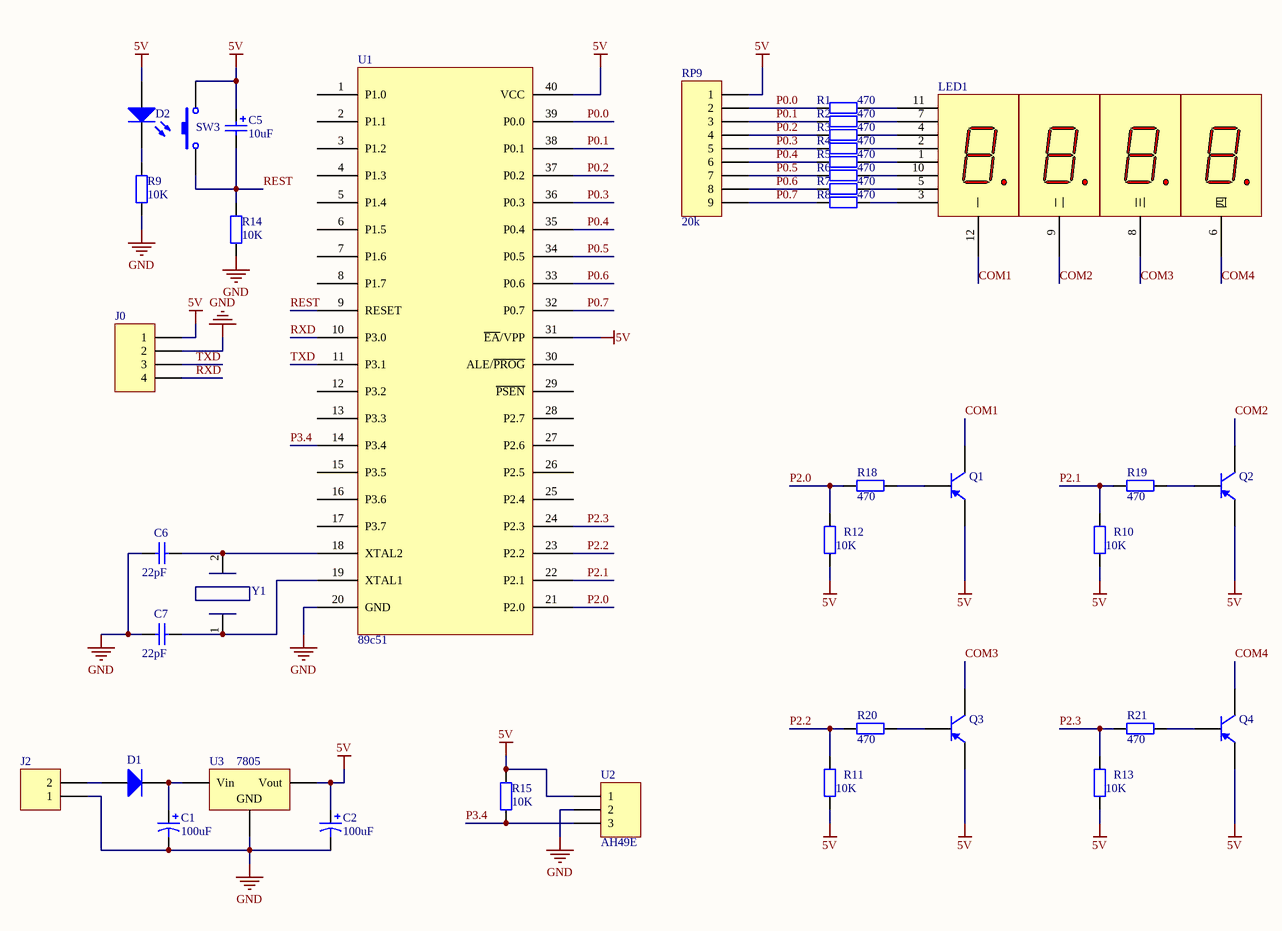
[diagram p0: MISC89328.SchDoc]
# Altium project MISC89328.PrjPcb
1 sheet, 39 parts. Net scope: global (net labels, ports and power ports of the same name join across sheets).
Board files: MISC89328.PcbDoc, MISC89328-28.PcbDoc

## Sheet MISC89328.SchDoc
size A3

### Parts
C1  100uF  [RB7.6-15]
C2  value 100uF  [RB7.6-15]  (hidden comment: Cap Pol1)
C5  value 10uF  [POLAR0.8]  (hidden comment: Cap Pol2)
C6  value 22pF  [RAD-0.3]  (hidden comment: Cap)
C7  value 22pF  [RAD-0.3]  (hidden comment: Cap)
D1  Diode 1N914  [DO-35]  (value not drawn)
D2  LED0  [LED-0]  (value not drawn)
J0  Header 4  [HDR1X4]  (value not drawn)
J2  Header 2  [HDR1X2]  (value not drawn)
LED1  Dpy Red-CA  [四位数码管]  (value not drawn)
Q1  2N3906  [TO-92A]  (value not drawn)
Q2  2N3906  [TO-92A]  (value not drawn)
Q3  2N3906  [TO-92A]  (value not drawn)
Q4  2N3906  [TO-92A]  (value not drawn)
R1  value 470  [AXIAL-0.4]  (hidden comment: Res2)
R2  value 470  [AXIAL-0.4]  (hidden comment: Res2)
R3  value 470  [AXIAL-0.4]  (hidden comment: Res2)
R4  value 470  [AXIAL-0.4]  (hidden comment: Res2)
R5  value 470  [AXIAL-0.4]  (hidden comment: Res2)
R6  value 470  [AXIAL-0.4]  (hidden comment: Res2)
R7  value 470  [AXIAL-0.4]  (hidden comment: Res2)
R8  value 470  [AXIAL-0.4]  (hidden comment: Res2)
R9  value 10K  [AXIAL-0.4]  (hidden comment: Res2)
R10  value 10K  [AXIAL-0.4]  (hidden comment: Res2)
R11  value 10K  [AXIAL-0.4]  (hidden comment: Res2)
R12  value 10K  [AXIAL-0.4]  (hidden comment: Res2)
R13  value 10K  [AXIAL-0.4]  (hidden comment: Res2)
R14  value 10K  [AXIAL-0.4]  (hidden comment: Res2)
R15  value 10K  [AXIAL-0.4]  (hidden comment: Res2)
R18  value 470  [AXIAL-0.4]  (hidden comment: Res2)
R19  value 470  [AXIAL-0.4]  (hidden comment: Res2)
R20  value 470  [AXIAL-0.4]  (hidden comment: Res2)
R21  value 470  [AXIAL-0.4]  (hidden comment: Res2)
RP9  20k  [HDR1X9]
SW3  SW-PB  [SPST-2]  (value not drawn)
U1  89c51  [89c51]
U2  AH49E  [HDR1X3]
U3  7805  [PCBComponent_1]
Y1  Component_1  [LC-HC-49S]  (value not drawn)

### Nets
5V: C2.1 C5.1 D2.1(A) J0.1 Q1.1(E) Q2.1(E) Q3.1(E) Q4.1(E) R10.1 R11.1 R12.1 R13.1 R15.2 RP9.1 SW3.2 U1.31(~{EA}/VPP) U1.40(VCC) U2.1 U3.3(Vout)
GND: C1.2 C2.2 C6.2 C7.2 J0.2 J2.1 R9.2 R14.2 U1.20(GND) U2.2 U3.2(GND)
COM1: LED1.12(一) Q1.3(C)
COM2: LED1.9(二) Q2.3(C)
COM3: LED1.8(三) Q3.3(C)
COM4: LED1.6(四) Q4.3(C)
P0.0: R1.1 RP9.2 U1.39(P0.0)
P0.1: R2.1 RP9.3 U1.38(P0.1)
P0.2: R3.1 RP9.4 U1.37(P0.2)
P0.3: R4.1 RP9.5 U1.36(P0.3)
P0.4: R5.1 RP9.6 U1.35(P0.4)
P0.5: R6.1 RP9.7 U1.34(P0.5)
P0.6: R7.1 RP9.8 U1.33(P0.6)
P0.7: R8.1 RP9.9 U1.32(P0.7)
P2.0: R12.2 R18.2 U1.21(P2.0)
P2.1: R10.2 R19.2 U1.22(P2.1)
P2.2: R11.2 R20.2 U1.23(P2.2)
P2.3: R13.2 R21.2 U1.24(P2.3)
P3.4: R15.1 U1.14(P3.4) U2.3
REST: C5.2 R14.1 SW3.1 U1.9(RESET)
RXD: J0.4 U1.10(P3.0)
TXD: J0.3 U1.11(P3.1)
NetC1_1: C1.1 D1.2(K) U3.1(Vin)
NetC6_1: C6.1 U1.18(XTAL2) Y1.2
NetC7_1: C7.1 U1.19(XTAL1) Y1.1
NetD1_1: D1.1(A) J2.2
NetD2_2: D2.2(K) R9.1
NetLED1_1: LED1.1 R5.2
NetLED1_2: LED1.2 R4.2
NetLED1_3: LED1.3 R8.2
NetLED1_4: LED1.4 R3.2
NetLED1_5: LED1.5 R7.2
NetLED1_7: LED1.7 R2.2
NetLED1_10: LED1.10 R6.2
NetLED1_11: LED1.11 R1.2
NetQ1_2: Q1.2(B) R18.1
NetQ2_2: Q2.2(B) R19.1
NetQ3_2: Q3.2(B) R20.1
NetQ4_2: Q4.2(B) R21.1

Not connected (* = marked no-connect by the designer): U1 1(P1.0) 2(P1.1) 3(P1.2) 4(P1.3) 5(P1.4) 6(P1.5) 7(P1.6) 8(P1.7) 12(P3.2) 13(P3.3) 15(P3.5) 16(P3.6) 17(P3.7) 25(P2.4) 26(P2.5) 27(P2.6) 28(P2.7) 29(~{PSEN}) 30(ALE/~{PROG})

### Library data of the parts
C1 C2 = Cap Pol1: Polarized Capacitor (Radial); Published: 8-Jun-2000; LatestRevisionDate: 17-Jul-2002; LatestRevisionNote: Re-released for DXP Platform.; PackageReference: RB7.6-15; PackageDescription: Polarized Capacitor (Radial); 2 Leads; Publisher: Altium Limited
  C1: Value: 100uF
C5 = Cap Pol2: Polarized Capacitor (Axial); Published: 8-Jun-2000; LatestRevisionDate: 17-Jul-2002; LatestRevisionNote: Re-released for DXP Platform.; PackageReference: POLAR0.8; PackageDescription: Polarized Capacitor; 2 Leads; Publisher: Altium Limited
C6 C7 = Cap: Capacitor; Published: 8-Jun-2000; LatestRevisionDate: 17-Jul-2002; LatestRevisionNote: Re-released for DXP Platform.; PackageReference: RAD-0.3; PackageDescription: Radial Cap, Thru-Hole; 2 Leads; 0.3 in Pin Spacing; Publisher: Altium Limited
D1 = Diode 1N914: High Conductance Fast Diode; Published: 8-Jun-2000; LatestRevisionDate: 17-Jul-2002; LatestRevisionNote: Re-released for DXP Platform.; DatasheetVersion: 1997; PackageReference: DO-35; PackageDescription: Diode, Axial; Body 3.8 x 1.9 mm (LxDia. max), Lead Dia. 0.53 mm (max); Code_JEDEC: DO-204-AH; ComponentLink1Description: Manufacturer Link; ComponentLink2Description: Datasheet; ComponentLink2URL: example.com/ds/1N%2F1N4448.pdf; Publisher: Altium Limited
D2 = LED0: Typical INFRARED GaAs LED; Published: 8-Jun-2000; LatestRevisionDate: 08-Jul-2005; LatestRevisionNote: Mech Layer 1 removed.; PackageReference: LED-0; PackageDescription: LED; 2 Leads; Publisher: Altium Limited
J0 = Header 4: Header, 4-Pin; LatestRevisionDate: 17-Jul-2002; LatestRevisionNote: Re-released for DXP Platform.; Publisher: Altium Limited
J2 = Header 2: Header, 2-Pin; LatestRevisionDate: 17-Jul-2002; LatestRevisionNote: Re-released for DXP Platform.; Publisher: Altium Limited
LED1 = Dpy Red-CA: 7.62 mm Black Surface HER 7-Segment Display: CA, RH DP; MinimumIntensity: 360 ucd; Note: IF = 5 mA; Colour: High Efficiency Red (HER); Note: Pins 1 and 6 are redundant Anodes.; Published: 8-Jun-2000; LatestRevisionDate: 17-Dec-2003; LatestRevisionNote: Schematic revised, PCB Footprint replaced.; DatasheetVersion: 19-Feb-2002; PackageVersion: 11-Feb-2002; PackageReference: A; PackageDescription: LED, 7-Segment Display, 7.62 mm, RHD; 10 Leads; Row Space 5.08 mm; Pitch 2.54 mm; ComponentLink1Description: Manufacturer Link; Publisher: Altium Limited
Q1-Q4 = 2N3906: PNP General Purpose Amplifier; Published: 8-Jun-2000; LatestRevisionDate: 15-Jan-2003; LatestRevisionNote: PCB Footprint 'BCY-W3/D4.7' replaced; DatasheetVersion: 1997; PackageVersion: Sep-1998; PackageReference: TO-92A; PackageDescription: TO, Flat Index; 3 In-Line, Axial Leads; Body Dia. 4.5mm; Leads 0.51 x 0.48 mm (max); ComponentLink1Description: Manufacturer Link; ComponentLink2Description: Datasheet; ComponentLink2URL: example.com/ds/2N%2F2N3906.pdf; Publisher: Altium Limited
R1-R15 R18-R21 = Res2: Resistor; Published: 8-Jun-2000; LatestRevisionDate: 17-Jul-2002; LatestRevisionNote: Re-released for DXP Platform.; PackageReference: AXIAL-0.4; PackageDescription: Axial Device, Thru-Hole; 2 Leads; 0.4 in Pin Spacing; Publisher: Altium Limited
RP9 = Header 9: Header, 9-Pin; LatestRevisionDate: 17-Jul-2002; LatestRevisionNote: Re-released for DXP Platform.; Publisher: Altium Limited
SW3 = SW-PB: Switch; Published: 24-Mar-1999; LatestRevisionDate: 17-Jul-2002; LatestRevisionNote: Re-released for DXP Platform.; PackageReference: SPST-2; PackageDescription: Switch; 2 Leads; Publisher: Altium Limited
U1 = Component_1
U2 = Header 3: Header, 3-Pin; LatestRevisionDate: 17-Jul-2002; LatestRevisionNote: Re-released for DXP Platform.; Publisher: Altium Limited
U3 = Volt Reg: Voltage Regulator; Published: 24-Mar-1999; LatestRevisionDate: 29-May-2009; LatestRevisionNote: IPC-7351 Footprint Added.; PackageReference: D2PAK; PackageDescription: 3-Pin Transistor Outline Package 2.54 mm Pitch, 15.1 mm Lead Span; Publisher: Altium Limited